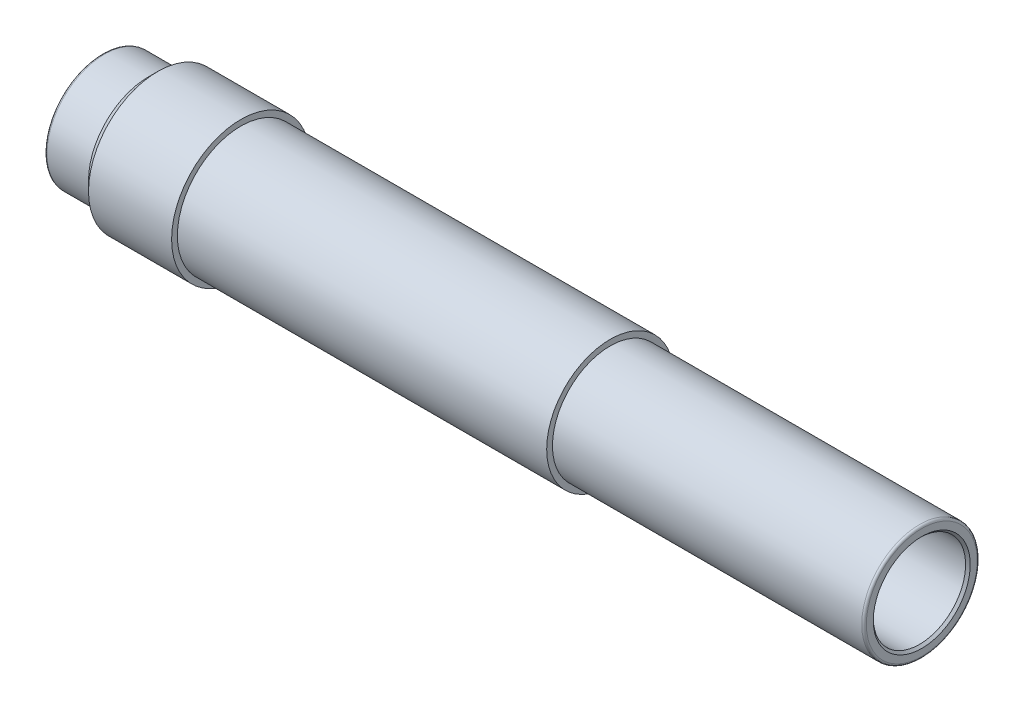
from build123d import *

# Parameters (mm, degrees)
FILLET1_R     = 1
CHAMFER1_SIZE = 1


with BuildPart() as part:
    # Sketch 1 → Revolve3 (revolve)
    with BuildSketch(Plane(origin=(0, 0, 0), x_dir=(1, 0, 0), z_dir=(0, 1, 0)), mode=Mode.PRIVATE) as revolve3_sk:
        Polygon((24, 30), (20, 26), (20, 25), (0, 25), (0, 20), (355, 20), (355, 25), (220, 25), (220, 27.5), (60, 27.5), (60, 30), align=None)
    revolve(revolve3_sk.sketch.rotate(Axis((20, 0, 0), (1, 0, 0)), 180), axis=Axis((20, 0, 0), (1, 0, 0)))

    # Fillet1
    fillet1_edges = [part.edges().sort_by_distance(p)[0] for p in [
        (355, 0, -25),
        (0, 0, -25),
    ]]
    fillet(fillet1_edges, radius=FILLET1_R)

    # Chamfer1
    chamfer1_edges = [part.edges().sort_by_distance(p)[0] for p in [
        (355, 0, -20),
    ]]
    chamfer(chamfer1_edges, length=CHAMFER1_SIZE)


solid = part.part
